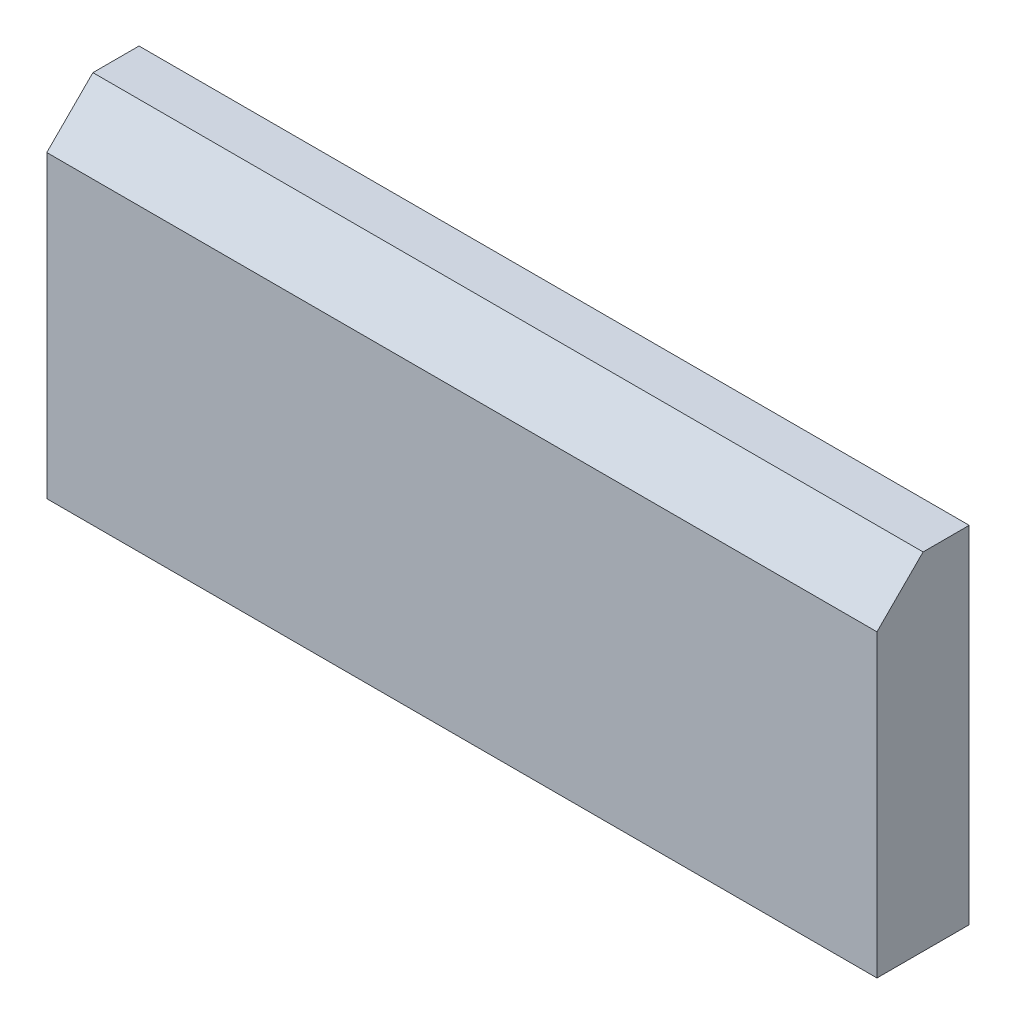
SolidWorks part; units mm, degrees
material "普通碳钢"
ref_plane "前视基准面" through (0, 0, 0) normal (0, 0, 1) x (1, 0, 0)
ref_plane "上视基准面" through (0, 0, 0) normal (0, 1, 0) x (1, 0, 0)
ref_plane "右视基准面" through (0, 0, 0) normal (1, 0, 0) x (0, 0, -1)
sketch "草图1" plane through (0, 0, 0) normal (0, 0, 1) x (1, 0, 0)
  line L0 (-344.0259, 0) -> (355.8889, 0) construction
  line L1 (0, 208.7882) -> (0, -239.6319) construction
  line L2 (-90, 0) -> (90, 0)
  line L3 (90, 0) -> (90, 75)
  line L4 (90, 75) -> (-90, 75)
  line L5 (-90, 75) -> (-90, 0)
  dimension "D1" = 180
  dimension "D2" = 75
extrude "凸台-拉伸1" add sketch "草图1" along normal blind 20
chamfer "倒角2" distance 10 angle 45 1 edges at (0, 75, 20)
